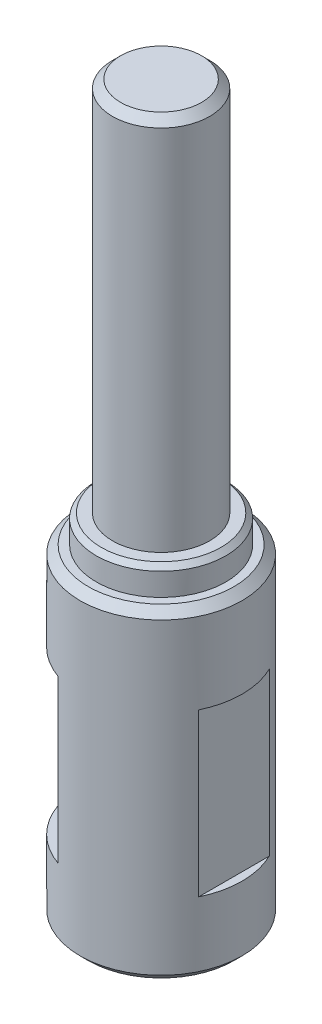
SolidWorks part; units mm, degrees
ref_plane "Front Plane" through (0, 0, 0) normal (0, 0, 1) x (1, 0, 0)
ref_plane "Top Plane" through (0, 0, 0) normal (0, 1, 0) x (1, 0, 0)
ref_plane "Right Plane" through (0, 0, 0) normal (1, 0, 0) x (0, 0, -1)
sketch "Sketch1" plane through (0, 0, 0) normal (0, 1, 0) x (1, 0, 0)
  circle A0 centre (0, 0) radius 3
  dimension "D1" = 6
extrude "Boss-Extrude1" add sketch "Sketch1" along normal blind 20.5
sketch "Sketch2" plane through (0, 20.5, 0) normal (0, 1, 0) x (1, 0, 0)
  circle A0 centre (0, 0) radius 4
  dimension "D1" = 8
extrude "Boss-Extrude2" add sketch "Sketch2" along normal blind 1.2
sketch "Sketch5" plane through (0, 21.7, 0) normal (0, 1, 0) x (1, 0, 0)
  circle A0 centre (0, 0) radius 3
  dimension "D1" = 6
extrude "Boss-Extrude3" add sketch "Sketch5" along normal blind 23.2
chamfer "Chamfer3" distance 0.5 angle 45 1 edges at (0, 44.9, 3)
sketch "Sketch6" plane through (0, 20.5, 0) normal (0, -1, 0) x (1, 0, 0)
  circle A0 centre (0, 0) radius 4 construction
  circle A1 centre (0, 0) radius 4
extrude "Boss-Extrude4" add sketch "Sketch6" along normal up to surface (20.5 mm away) up to face at (0, 0, 3)
chamfer "Chamfer4" distance 0.3 angle 45 1 edges at (0, 21.7, 4)
sketch "Sketch9" plane through (0, 0, 0) normal (0, -1, 0) x (1, 0, 0)
  circle A0 centre (0, 0) radius 5
  dimension "D1" = 10
extrude "Boss-Extrude5" add sketch "Sketch9" against normal blind 20
chamfer "Chamfer5" distance 0.5 angle 45 2 edges at (0, 20, -5) (0, 0, -5)
sketch "Sketch10" plane through (0, 0, 0) normal (0, 0, 1) x (1, 0, 0)
  line L0 (0, 0) -> (0, 50000) construction
  line L1 (5, 0.5) -> (5, 19.5) construction
  line L2 (4.5, 14.5) -> (5.5, 14.5)
  line L3 (4.5, 14.5) -> (4.5, 4.5)
  line L4 (4.5, 4.5) -> (5.5, 4.5)
  line L5 (5.5, 14.5) -> (5.5, 4.5)
  line L6 (4.5, 14.5) -> (5.5, 4.5) construction
  line L7 (4.5, 4.5) -> (5.5, 14.5) construction
  line L8 (-4.5, 0) -> (4.5, 0) construction
  point P3 (5, 9.5)
  dimension "D1" = 10
  dimension "D2" = 0.5
  dimension "D3" = 9.5
extrude "Cut-Extrude2" cut sketch "Sketch10" against normal mid plane 20
pattern_circular "CirPattern2" count 2 every 135 about axis through (0, 44.9, 0) along (0, -1, 0) of "Cut-Extrude2"
